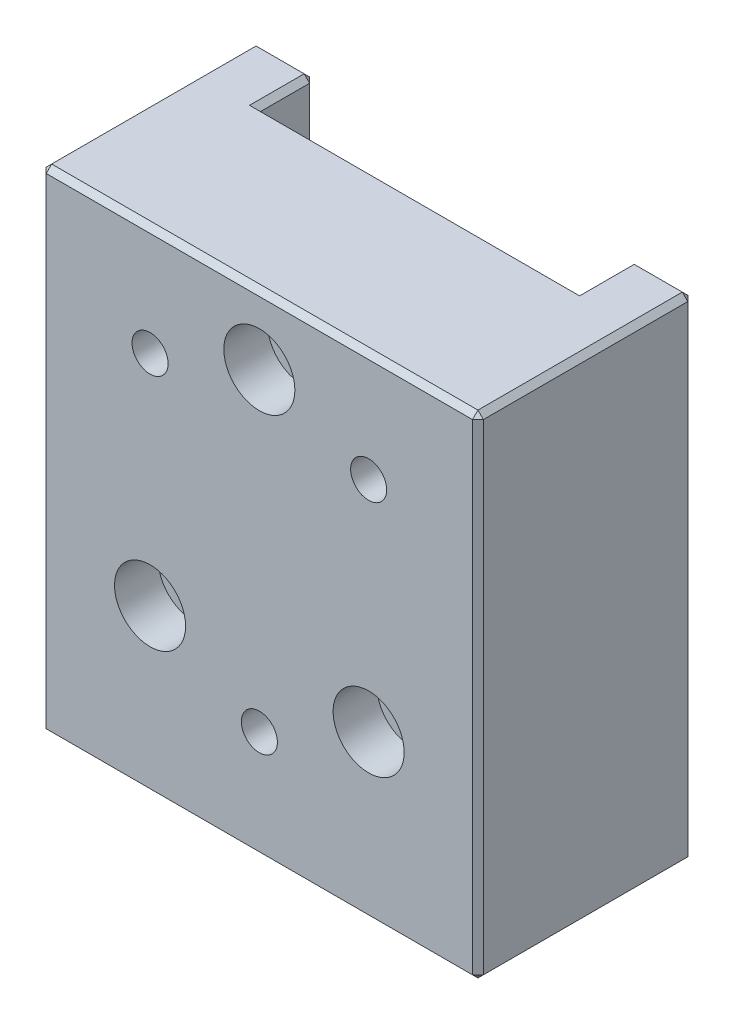
SolidWorks part; units mm, degrees
material "6061 合金"
ref_plane "前视基准面" through (0, 0, 0) normal (0, 0, 1) x (1, 0, 0)
ref_plane "上视基准面" through (0, 0, 0) normal (0, 1, 0) x (1, 0, 0)
ref_plane "右视基准面" through (0, 0, 0) normal (1, 0, 0) x (0, 0, -1)
sketch "草图1" plane through (0, 0, 0) normal (0, 0, 1) x (1, 0, 0)
  line L1 (-20, 22.5) -> (20, 22.5)
  line L2 (-20, 22.5) -> (-20, -22.5)
  line L3 (-20, -22.5) -> (20, -22.5)
  line L4 (20, 22.5) -> (20, -22.5)
  line L5 (-20, 22.5) -> (20, -22.5) construction
  line L6 (-20, -22.5) -> (20, 22.5) construction
  point P0 (0, 0)
  dimension "D1" = 45
  dimension "D2" = 40
extrude "凸台-拉伸1" add sketch "草图1" along normal mid plane 14.7
hole_wizard "M3 六角凹头螺钉的柱形沉头孔1" positions "草图3" profile "草图4" counterbore size "M3" standard "ISO" end condition through all
sketch "草图3" plane through (0, 0, 7.35) normal (0, 0, 1) x (1, 0, 0)
  line L0 (-20, -22.5) -> (20, -22.5) construction
  point P0 (0, 16.2)
  point P2 (-10, -7.5)
  point P4 (10, -7.5)
  dimension "D1" = 23.7
  dimension "D2" = 15
sketch "草图4" plane through (0, 16.2, 7.35) normal (1, 0, 0) x (0, -1, 0)
  line L0 (0, 0) -> (0, 14.7)
  line L1 (0, 14.7) -> (1.7, 14.7)
  line L3 (1.7, 14.7) -> (1.7, 4)
  line L4 (1.7, 4) -> (3.25, 4)
  line L5 (3.25, 4) -> (3.25, 0)
  line L7 (3.25, 0) -> (0, 0)
  line L11 (0, -6.35) -> (0, 107.95) construction
  dimension "通孔孔直径" = 3.4
  dimension "通孔孔深度" = 14.7
  dimension "柱形沉头孔直径" = 6.5
  dimension "柱形沉头孔深度" = 4
sketch "草图5" plane through (0, 0, -7.35) normal (0, 0, -1) x (-1, 0, 0)
  line L0 (-20, 22.5) -> (20, 22.5) construction
  line L1 (-20, 22.5) -> (-14.6, 22.5)
  line L2 (-20, 22.5) -> (-20, -22.5)
  line L3 (-20, -22.5) -> (-14.6, -22.5)
  line L4 (-14.6, 22.5) -> (-14.6, -22.5)
  line L5 (20, -22.5) -> (-20, -22.5) construction
  line L6 (0, 8.085) -> (0, -8.085) construction
  line L7 (14.6, 22.5) -> (20, 22.5)
  line L8 (14.6, 22.5) -> (14.6, -22.5)
  line L9 (14.6, -22.5) -> (20, -22.5)
  line L10 (20, 22.5) -> (20, -22.5)
  line L11 (20, 22.5) -> (20, -22.5) construction
  dimension "D3" = 29.2
  dimension "D4" = 14.6
extrude "凸台-拉伸2" add sketch "草图5" along normal blind 5
hole_wizard "M4 螺纹孔2" positions "草图7" profile "草图8" tap size "M4" standard "ISO" end condition through all
sketch "草图7" plane through (0, 0, 7.35) normal (0, 0, 1) x (1, 0, 0)
  line L1 (0, 22.5) -> (0, -22.5) construction
  line L2 (20, 22.5) -> (-20, 22.5) construction
  line L3 (-20, -22.5) -> (20, -22.5) construction
  point P0 (10, 12.5)
  point P3 (-10, 12.5)
  point P6 (0, -12.5)
  dimension "D1" = 20
  dimension "D2" = 25
  dimension "D3" = 10
sketch "草图8" plane through (10, 12.5, 7.35) normal (1, 0, 0) x (0, -1, 0)
  line L0 (0, 0) -> (0, 19.7)
  line L1 (0, 19.7) -> (1.65, 19.7)
  line L2 (1.65, 19.7) -> (1.65, 0)
  line L5 (1.65, 0) -> (0, 0)
  line L11 (0, -6.35) -> (0, 107.95) construction
  dimension "通孔螺纹孔钻头直径" = 3.3
  dimension "通孔螺纹孔钻头深度" = 19.7
cosmetic thread "孔螺蚊线1" parameters "D2"=4
cosmetic thread "孔螺蚊线2" parameters "D2"=4
cosmetic thread "孔螺蚊线3" parameters "D2"=4
chamfer "倒角1" distance 0.5 angle 45 22 edges at (0, 22.5, 7.35) (-20, 22.5, -2.5) (-17.3, 22.5, -12.35) (-14.6, 22.5, -9.85) (0, 22.5, -7.35) (14.6, 22.5, -9.85) (17.3, 22.5, -12.35) (20, 22.5, -2.5) (0, -22.5, 7.35) (20, 0, 7.35) (20, -22.5, -2.5) (20, 0, -12.35) (17.3, -22.5, -12.35) (14.6, 0, -12.35) (14.6, -22.5, -9.85) (0, -22.5, -7.35) (-14.6, -22.5, -9.85) (-14.6, 0, -12.35) (-17.3, -22.5, -12.35) (-20, 0, -12.35) (-20, -22.5, -2.5) (-20, 0, 7.35)
